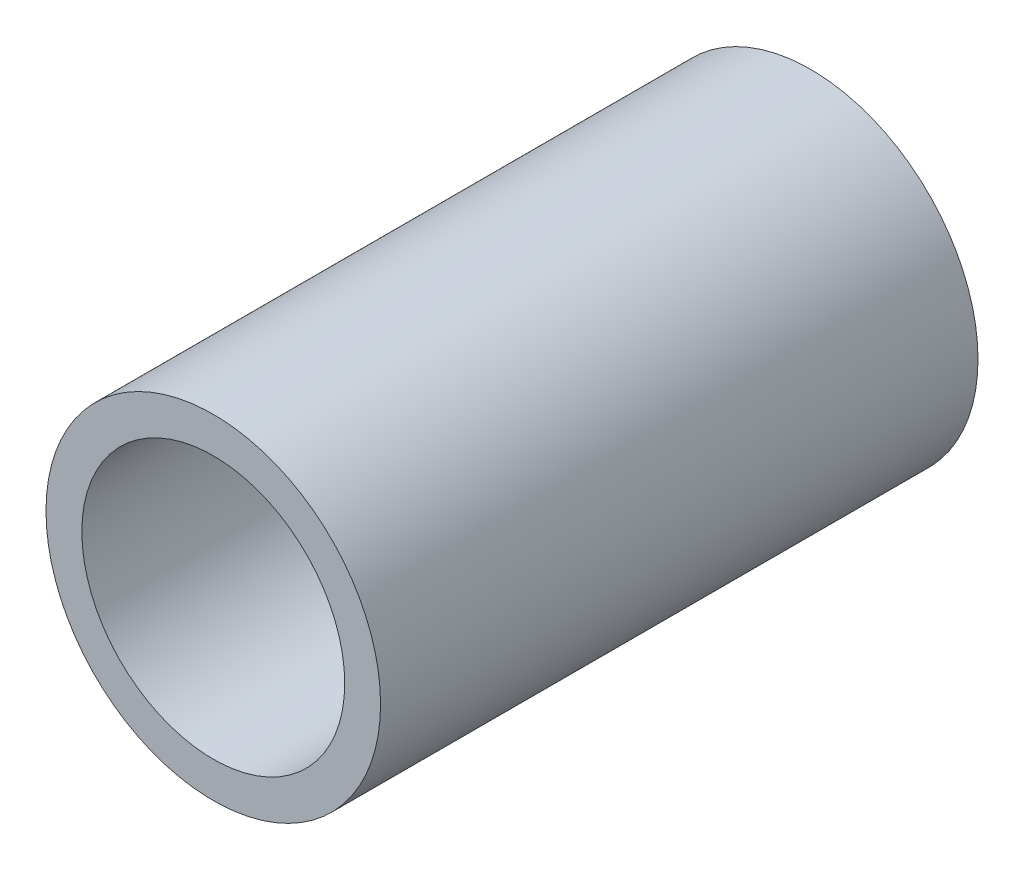
from build123d import *

# Parameters (mm, degrees)
SKETCH_1_R      = 28
SKETCH_1_R_2    = 22
EXTRUDE_1_DEPTH = 50


with BuildPart() as part:
    # 草图1 → 凸台-拉伸1 (new, symmetric)
    with BuildSketch(Plane.XY):
        Circle(SKETCH_1_R)
        Circle(SKETCH_1_R_2, mode=Mode.SUBTRACT)
    extrude(amount=EXTRUDE_1_DEPTH, both=True)


solid = part.part
